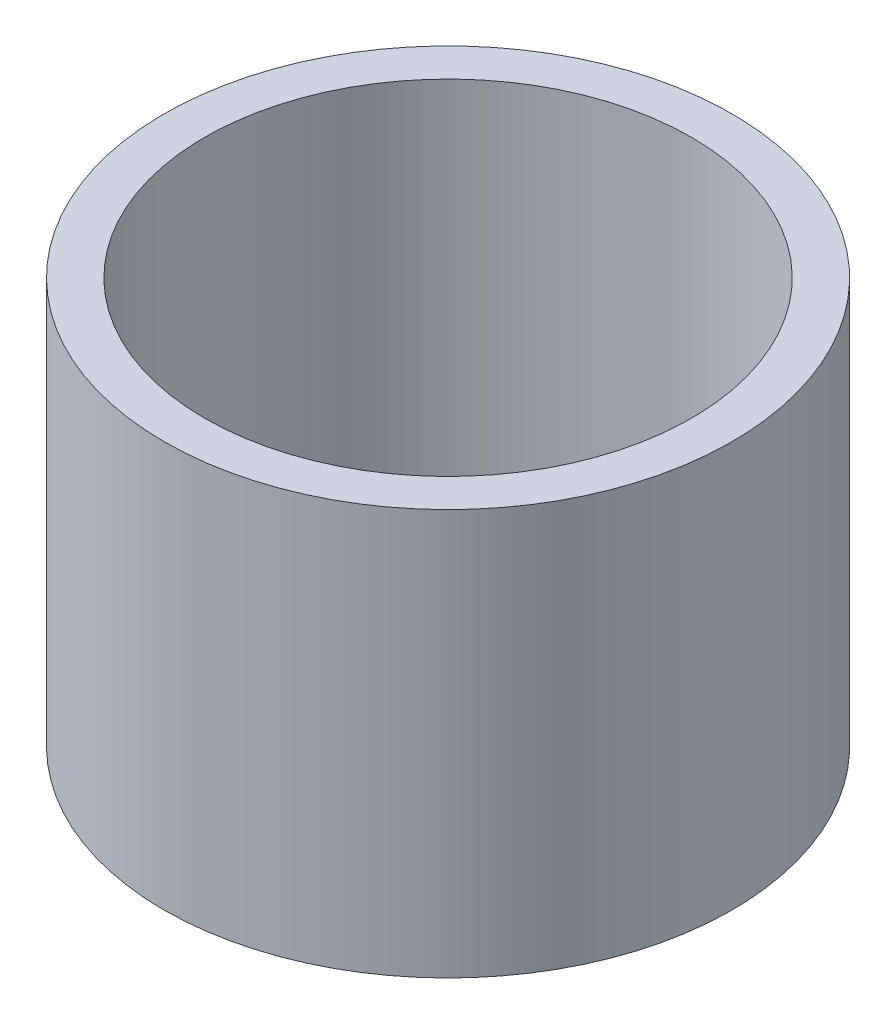
from build123d import *

# Parameters (mm, degrees)
SKETCH1_R           = 70
SKETCH1_R_2         = 60
BOSS_EXTRUDE1_DEPTH = 100


with BuildPart() as part:
    # Sketch1 → Boss-Extrude1 (new body)
    with BuildSketch(Plane(origin=(0, 0, 0), x_dir=(1, 0, 0), z_dir=(0, 1, 0))):
        with Locations(Location((0, 0, 0), (0, 0, 270))):
            Circle(SKETCH1_R)
        with Locations(Location((0, 0, 0), (0, 0, 270))):
            Circle(SKETCH1_R_2, mode=Mode.SUBTRACT)
    extrude(amount=BOSS_EXTRUDE1_DEPTH)


solid = part.part
